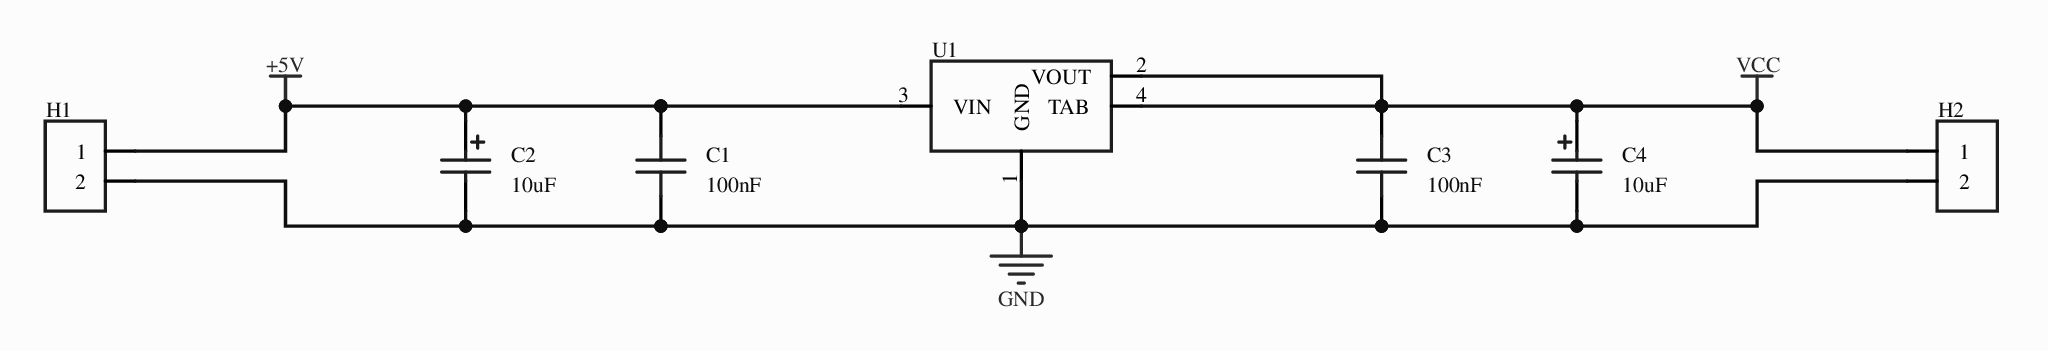
[diagram p0: MISC52016-3.schdoc]
# Altium project MISC52016-2.PrjPcb
1 sheet, 7 parts. Net scope: global (net labels, ports and power ports of the same name join across sheets).
Board file: MISC52016.pcbdoc

## Sheet MISC52016-3.schdoc
size 297 x 209 mm; Version: V1.0; @Project Name: MISC52016; @Update Date: 2026-03-13; @Create Date: 2026-03-13; @Board Name: MISC52016; @Create Time: 20:40:58; @Page Count: 1; @Page No: 1; @Schematic Name: MISC52016; @Update Time: 20:40:58; Size: A4

### Parts
C1  100nF  [C0603]
C2  10uF  [C_Ele_SMD_3x5.4mm]
C3  100nF  [C0603]
C4  10uF  [C_Ele_SMD_3x5.4mm]
H1  (no value)  [HDR-TH_2P-P2.54-V-F]
H2  (no value)  [HDR-TH_2P-P2.54-V-F]
U1  (no value)  [SOT_223]

### Nets
+5V: C1.2 C2.1 H1.1 U1.3(VIN)
GND: C1.1 C2.2 C3.1 C4.2 H1.2 H2.2 U1.1(GND)
VCC: C3.2 C4.1 H2.1 U1.2(VOUT) U1.4(TAB)

### Library data of the parts
C1 C3 = CAP_0603: Symbol: Capacitance; ConvertToPcb: yes; ModelId: ac125912035d415993ca9572d50418b10819f05c4eef4c71ace90d822a990e87; ModelName: C0603_L1.6-W0.8-H0.8; ModelTransform: 62.992,31.496,0,0,0,0,0,0,0; Device: CAP_0603; AddInBom: yes; Supplier Footprint: 0603; FootprintName: C0603; Value: 100nF
C2 C4 = C_Ele_SMD_3x5.4mm: Symbol: CAP; AddInBom: yes; ModelId: 0132c3d3fdbf4fd987f710a97e7a5b5d0819f05c4eef4c71ace90d822a990e87; ModelName: CAP-SMD_BD3.0-L3.3-W3.3-H5.3; ModelTransform: 129.9,149.58,209.06,-90,0,0,0,0,0; Device: C_Ele_SMD_3x5.4mm; Supplier Footprint: SMD,3x5.4mm; ConvertToPcb: yes; FootprintName: C_Ele_SMD_3x5.4mm; Value: 10uF
H1 H2 = HDR-F_2.54_1x2P: Symbol: Header-Female-2.54_1x2; ConvertToPcb: yes; ModelId: a9450ef445564560a104363b9aacde4e0819f05c4eef4c71ace90d822a990e87; ModelName: HDR-TH_2P-P2.54-F-LI-1X2P; ModelTransform: 215.7476,98.425,0,0,0,0,0,0,-129.921; Device: HDR-F_2.54_1x2P; AddInBom: yes; SupplierPart: C49661; Supplier Footprint: 插件; FootprintName: HDR-TH_2P-P2.54-V-F
U1 = AMS1117: Symbol: AMS1117_OLD; AddInBom: yes; ModelId: 925194bf9823436183a3e0b978a8d0760819f05c4eef4c71ace90d822a990e87; ModelName: SOT-223-4P_L6.5-W3.5-H1.6-LS7.0-P2.30; ModelTransform: 279.84,255.85,68.86,90,0,0,0,0,0; Device: AMS1117; ConvertToPcb: yes; FootprintName: SOT_223